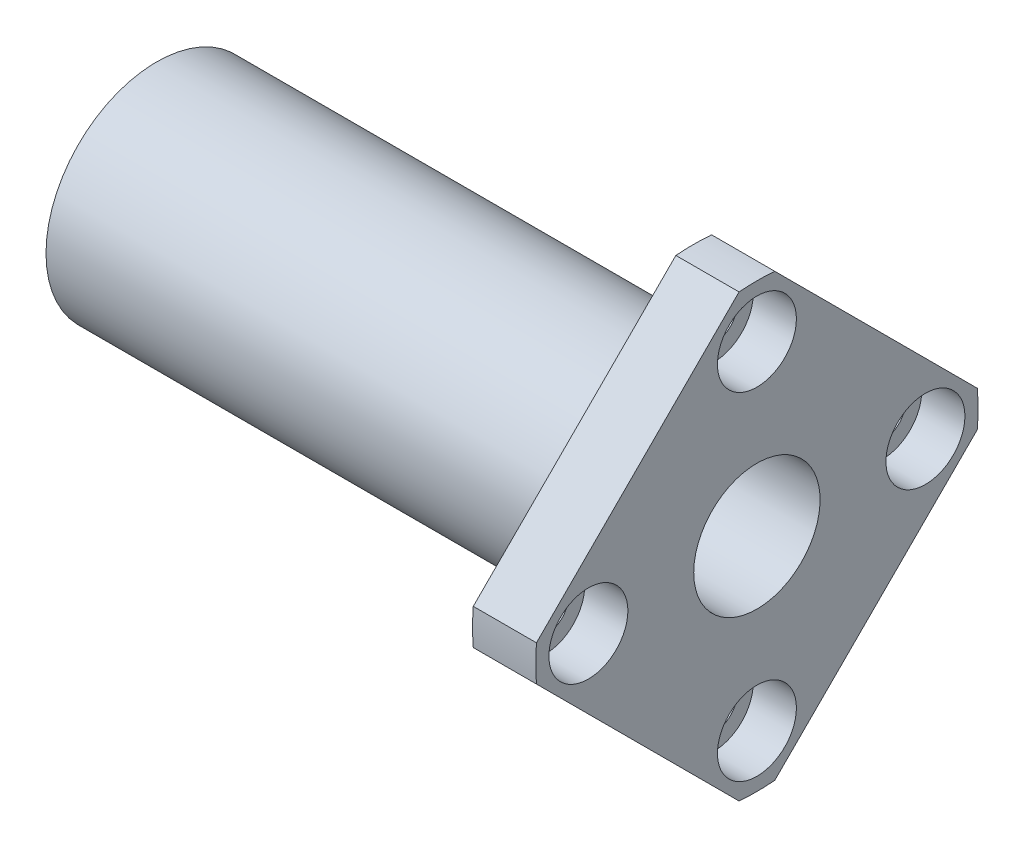
from build123d import *

# Parameters (mm, degrees)
SKETCH1_R                      = 10.5
SKETCH1_R_2                    = 6
BOSS_EXTRUDE1_DEPTH            = 28.5
BOSS_EXTRUDE2_START            = -6
SKETCH2_R                      = 21
SKETCH2_R_2                    = 6
BOSS_EXTRUDE2_DEPTH            = 6
F_7_5_7_5_DIAMETER_HOLE1_D     = 7.5
F_7_5_7_5_DIAMETER_HOLE1_DEPTH = 4.1
F_4_5_4_5_DIAMETER_HOLE1_D     = 4.5
CIRPATTERN1_COUNT              = 4
CUT_EXTRUDE1_START             = -6
SKETCH7_OUTSIDE_W              = 60.464
SKETCH7_OUTSIDE_H              = 60.464
CUT_EXTRUDE1_DEPTH             = 6


with BuildPart() as part:
    # Sketch1 → Boss-Extrude1 (new, symmetric)
    with BuildSketch(Plane(origin=(0, 0, 0), x_dir=(0, 0, -1), z_dir=(1, 0, 0))):
        with Locations(Location((0, 0, 0), (0, 0, 180))):
            Circle(SKETCH1_R)
        with Locations(Location((0, 0, 0), (0, 0, 180))):
            Circle(SKETCH1_R_2, mode=Mode.SUBTRACT)
    extrude(amount=BOSS_EXTRUDE1_DEPTH, both=True)

    # Sketch2 → Boss-Extrude2 (add)
    with BuildSketch(Plane(origin=(28.5, 0, 0), x_dir=(0, 0, -1), z_dir=(1, 0, 0)).offset(BOSS_EXTRUDE2_START)):
        Circle(SKETCH2_R)
        with Locations(Location((0, 0, 0), (0, 0, 180))):
            Circle(SKETCH2_R_2, mode=Mode.SUBTRACT)
    extrude(amount=BOSS_EXTRUDE2_DEPTH)

    # Ø7.5 (7.5) Diameter Hole1
    with Locations(Plane(origin=(28.5, 0, 0), x_dir=(0, 0, -1), z_dir=(1, 0, 0))):
        with Locations((0, 16)):
            f_7_5_7_5_diameter_hole1 = Hole(F_7_5_7_5_DIAMETER_HOLE1_D / 2, depth=F_7_5_7_5_DIAMETER_HOLE1_DEPTH)

    # Ø4.5 (4.5) Diameter Hole1 (through all)
    with Locations(Plane(origin=(24.4, 0, 0), x_dir=(0, 0, -1), z_dir=(1, 0, 0))):
        with Locations((0, 16)):
            f_4_5_4_5_diameter_hole1 = Hole(F_4_5_4_5_DIAMETER_HOLE1_D / 2)

    # CirPattern1: Ø7.5 (7.5) Diameter Hole1, Ø4.5 (4.5) Diameter Hole1 ×4 about axis
    cirpattern1_axis = Axis((0, 0, 0), (1, 0, 0))
    add([f_7_5_7_5_diameter_hole1.rotate(cirpattern1_axis, i * 360 / CIRPATTERN1_COUNT) for i in range(1, CIRPATTERN1_COUNT)], mode=Mode.SUBTRACT)
    add([f_4_5_4_5_diameter_hole1.rotate(cirpattern1_axis, i * 360 / CIRPATTERN1_COUNT) for i in range(1, CIRPATTERN1_COUNT)], mode=Mode.SUBTRACT)

    # Sketch7 outside → Cut-Extrude1 (cut)
    with BuildSketch(Plane(origin=(28.5, 0, 0), x_dir=(0, 0, -1), z_dir=(1, 0, 0)).offset(CUT_EXTRUDE1_START)):
        Rectangle(SKETCH7_OUTSIDE_W, SKETCH7_OUTSIDE_H)
        Polygon((0, 22.627416998), (-22.627416998, 0), (0, -22.627416998), (22.627416998, 0), align=None, mode=Mode.SUBTRACT)
    extrude(amount=CUT_EXTRUDE1_DEPTH, mode=Mode.SUBTRACT)


solid = part.part
